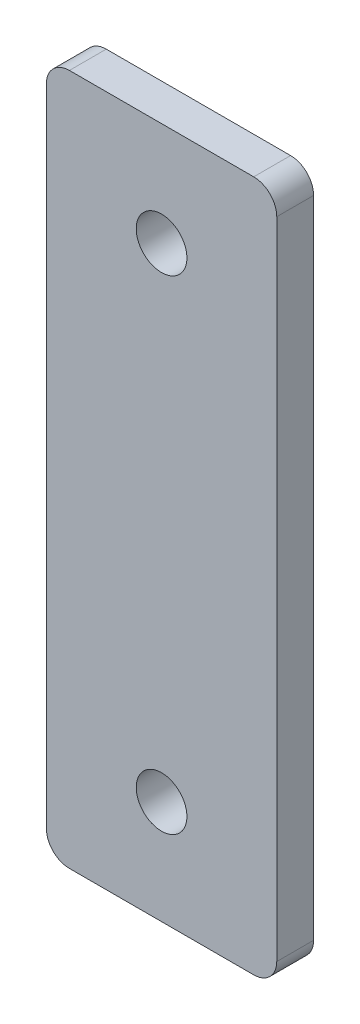
SolidWorks part; units mm, degrees
material "Q235B"
ref_plane "Front Plane" through (0, 0, 0) normal (0, 0, 1) x (1, 0, 0)
ref_plane "Top Plane" through (0, 0, 0) normal (0, 1, 0) x (1, 0, 0)
ref_plane "Right Plane" through (0, 0, 0) normal (1, 0, 0) x (0, 0, -1)
sketch "Sketch1" plane through (0, 0, 0) normal (0, 0, 1) x (1, 0, 0)
  line L1 (20, -75) -> (-20, -75)
  line L2 (25, -70) -> (25, 70)
  line L3 (20, 75) -> (-20, 75)
  line L4 (-25, -70) -> (-25, 70)
  line L5 (25, -75) -> (-25, 75) construction
  line L6 (25, 75) -> (-25, -75) construction
  arc A0 (-20, -75) -> (-25, -70) centre (-20, -70) cw
  arc A1 (25, 70) -> (20, 75) centre (20, 70) ccw
  arc A2 (20, -75) -> (25, -70) centre (20, -70) ccw
  arc A3 (-20, 75) -> (-25, 70) centre (-20, 70) ccw
  point P0 (0, 0)
  dimension "D3" = 5
  dimension "D1" = 150
  dimension "D2" = 50
extrude "Boss-Extrude1" add sketch "Sketch1" along normal blind 8
hole_wizard "Ø11.0 (11) Diameter Hole5" positions "Sketch2" profile "Sketch3" hole size "Ø11.0" standard "GB" end condition up to next
sketch "Sketch2" plane through (0, 0, 8) normal (0, 0, 1) x (1, 0, 0)
  line L0 (0, 0) -> (0, 52.5) construction
  line L2 (0, 0) -> (25, 0) construction
  line L3 (25, -70) -> (25, 70) construction
  point P0 (0, 52.5)
  point P15 (0, -52.5)
  dimension "D1" = 105
sketch "Sketch3" plane through (0, 52.5, 8) normal (1, 0, 0) x (0, -1, 0)
  line L0 (0, 0) -> (0, 8)
  line L1 (0, 8) -> (5.5, 8)
  line L2 (5.5, 8) -> (5.5, 0)
  line L5 (5.5, 0) -> (0, 0)
  line L11 (0, -6.35) -> (0, 107.95) construction
  dimension "通孔孔直径" = 11
  dimension "通孔孔深度" = 8
